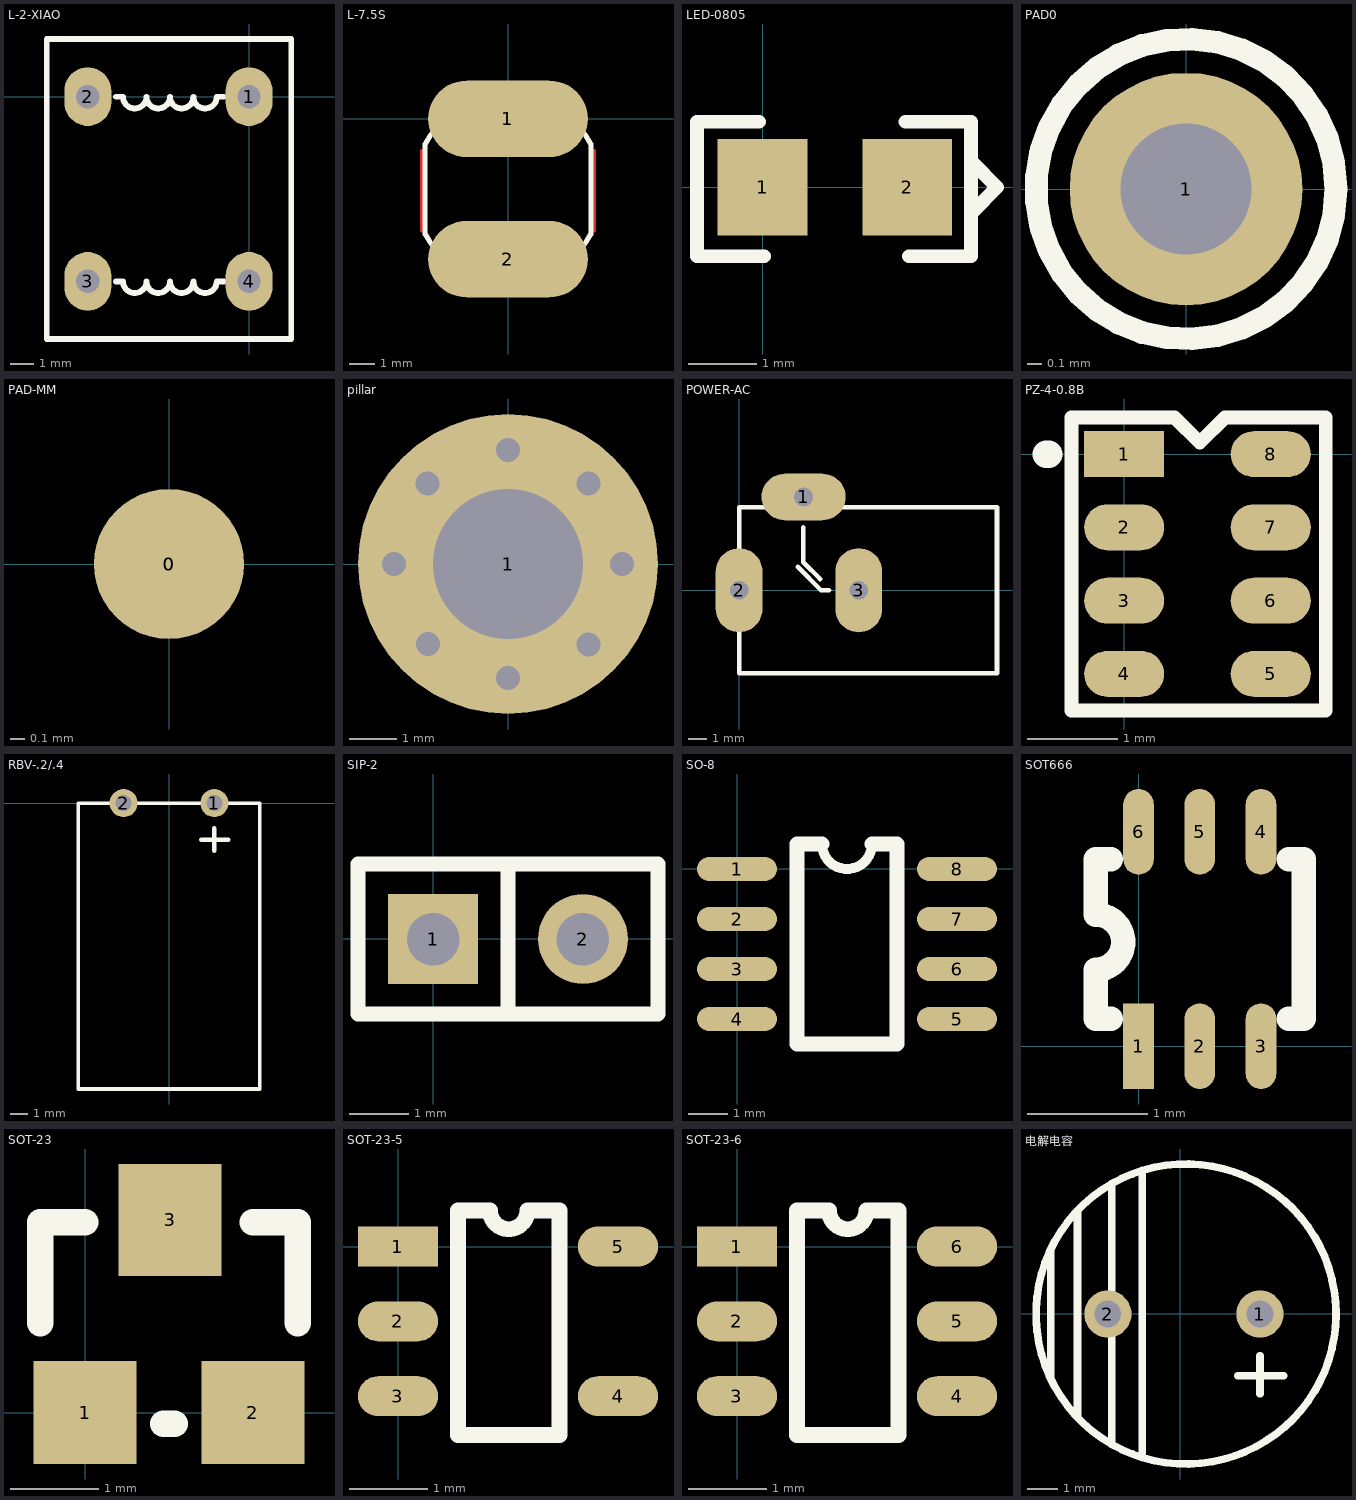
[diagram p0: the footprints below, top view; thin cyan lines are the x and y axes]
# Altium footprint library MISC103926-16.PcbLib: 32 footprints (part 2 of 2)
Each footprint in its own frame and in the unit in brackets; x right, y up, seen from the top. Pads: shape width x height; smd on the part's side, far side on the other; paste and mask are expansions set on the pad; w line width, h text height; cw(c..) or ccw(c..) is an arc to the next point about the centre after c.

## L-2-XIAO [mil]
height 270.08
pads (4):
  oval 80x100 hole 40: 1(0,0) 2(-275,0) 3(-275,-315) 4(0,-315)
Top Overlay:
  lines w10: -227,-315 -215,-315 ccw(c-195,-315) -175,-315 ccw(c-155,-315) -135,-315 ccw(c-115,-315) -95,-315 ccw(c-75,-315) -55,-315 -43,-315 ; -227,0 -215,0 ccw(c-195,0) -175,0 ccw(c-155,0) -135,0 ccw(c-115,0) -95,0 ccw(c-75,0) -55,0 -43,0 ; -345,-413.39 -345,98.43 72,98.43 72,-413.39 -345,-413.39

## L-7.5S [mil]
pads (2):
  oval 250x120 smd: 1(0,0) 2(0,-220)
Top Layer:
  lines w6: -135,-175 -135,-50 ; 135,-175 135,-50
Top Overlay:
  lines w8: -130,-181 -130,-40 ; -129.58,-180.77 ccw(c0,-110) 129.58,-180.77 ; -129.58,-39.23 cw(c0,-110) 129.58,-39.23 ; 130,-181 130,-40

## LED-0805 [mil]
height 270.08
pads (2):
  rect 52x56 smd: 1(0,0) 2(84,0)
Top Overlay:
  lines w8: -2,38 -38,38 -38,-40 1,-40 ; 83,38 121,38 121,-40 85,-40 ; 122,-14 136,0 122,14

## PAD0 [mil]
height 68.9
pads (1):
  round 62 hole 35: 1(0,0)
Top Overlay:
  circle w6.06: c0,0 r40

## PAD-MM [mil]
height 68.9
pads (2):
  round 40 smd: 0(0,0)
  round 80 on Top Solder: 0(0,0)

## pillar [mil]
height 68.9
pads (1):
  round 250 hole 125: 1(0,0)
via -95,0 diameter 40 hole 20
via 0,95 diameter 40 hole 20
via 0,-95 diameter 40 hole 20
via 95,0 diameter 40 hole 20
via 67.12,67.12 diameter 40 hole 20
via -67.16,67.16 diameter 40 hole 20
via -66.82,-66.82 diameter 40 hole 20
via 67.16,-67.16 diameter 40 hole 20

## POWER-AC [mil]
height 38
pads (3):
  oval 180x100 hole 40: 1(137.8,199.37)
  oval 100x180 hole 40: 2(0,0) 3(255.91,0)
Top Overlay:
  lines w10: 125,50 175,0 192,0 ; 137,134 137,60 173,24 ; -18.48,-59.06 20.89,-59.06 20.89,59.05 -18.48,59.05 -18.48,-59.06 ; 0,-177.17 0,177.16 551.18,177.16 551.18,-177.17 0,-177.17 ; 78.74,177.16 78.74,216.54 196.85,216.54 196.85,177.16 78.74,177.16 ; 235.43,-59.43 274.8,-59.43 274.8,58.68 235.43,58.68 235.43,-59.43
Mechanical 1:
  lines w10: -21,-60.63 -21,59.37 19,59.37 19,-60.63 -21,-60.63 ; 77.8,179.37 77.8,219.37 197.8,219.37 197.8,179.37 77.8,179.37 ; 237,-61 237,59 277,59 277,-61 237,-61

## PZ-4-0.8B [mil]
height 270.08
pads (8):
  rect 35x20 smd: 1(0,0)
  oval 35x20 smd: 2(0,-32) 3(0,-64) 4(0,-96) 5(64,-96) 6(64,-64) 7(64,-32) 8(64,0)
Top Overlay:
  lines w6: -23,-112 -23,16 22,16 33,5 44,16 88,16 88,-112 -23,-112
  lines w12: -34,0 -33,0

## RBV-.2/.4 [mil]
height 38
pads (2):
  round 62 hole 35: 1(100,0) 2(-100,0)
Top Overlay:
  lines w8: -200,-629.92 200,-629.92 200,0 -200,0 -200,-629.92
  lines w10: 71,-81 131,-81 ; 100,-105 100,-55

## SIP-2 [mil]
height 270.08
pads (2):
  rect 60x60 hole 35: 1(0,0)
  round 60 hole 35: 2(100,0)
Top Overlay:
  lines w10: 50,-50 50,50 ; -50,-50 150,-50 150,50 -50,50 -50,-50

## SO-8 [mil]
height 270.08
pads (8):
  oval 80x24 smd: 1(0,0) 2(0,-50) 3(0,-100) 4(0,-150) 5(220,-150) 6(220,-100) 7(220,-50) 8(220,0)
Top Overlay:
  lines w10: 85,25 ccw(c110,25) 135,25
  lines w15: 85,25 60,25 60,-175 160,-175 160,25 135,25

## SOT666 [mil]
height 270.08
pads (6):
  rect 10x28 smd: 1(0,0)
  oval 10x28 smd: 2(20,0) 3(40,0) 4(40,70) 5(20,70) 6(0,70)
Top Overlay:
  lines w8: -9,9 -14,9 -14,25 ccw(c-14,34) -14,43 -14,61 -9,61 ; 49,9 54,9 54,61 49,61

## SOT-23 [mil]
height 270.08
pads (3):
  rect 46x46 smd: 1(0,0) 2(75,0)
  rect 46x50 smd: 3(38,86)
Top Overlay:
  lines w12: -20,40 -20,85 0,85 ; 35,-5 40,-5 ; 75,85 95,85 95,40

## SOT-23-5 [mil]
height 270.08
pads (5):
  rect 40x20 smd: 1(0,0)
  oval 40x20 smd: 2(0,-37.4) 3(0,-74.8) 4(110,-74.8) 5(110,0)
Top Overlay:
  lines w7.87: 30,18 30,-94.2 80.7,-94.2 80.7,18 ; 46,18 ccw(c55.35,18) 64.7,18
  lines w8: 30,18 46,18 ; 64.7,18 80.7,18

## SOT-23-6 [mil]
height 270.08
pads (6):
  rect 40x20 smd: 1(0,0)
  oval 40x20 smd: 2(0,-37.4) 3(0,-74.8) 4(110,-74.8) 5(110,-37.4) 6(110,0)
Top Overlay:
  lines w7.87: 30,18 30,-94.2 80.7,-94.2 80.7,18 ; 46,18 ccw(c55.35,18) 64.7,18
  lines w8: 30,18 46,18 ; 64.7,18 80.7,18

## 电解电容 [mil]
height 630
pads (2):
  round 62 hole 35: 1(105,0) 2(-95,0)
Top Overlay:
  circle w10: c7.71,0 r197.29
  lines w10: -170,-85 -170,85 ; -135,-135 -135,135 ; -90,-170 -90,170 ; -50,-185 -50,185 ; 76,-81 136,-81 ; 105,-105 105,-55